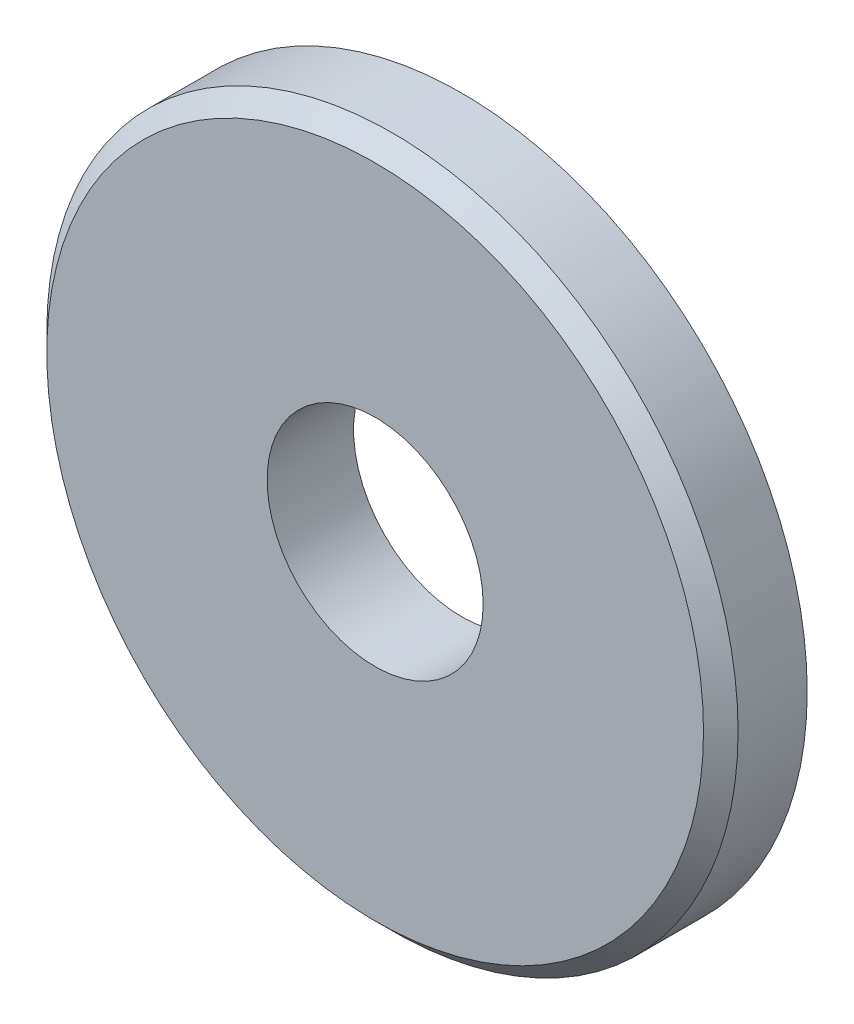
SolidWorks part; units mm, degrees
material "1023 碳钢板 (SS)"
ref_plane "前视基准面" through (0, 0, 0) normal (0, 0, 1) x (1, 0, 0)
ref_plane "上视基准面" through (0, 0, 0) normal (0, 1, 0) x (1, 0, 0)
ref_plane "右视基准面" through (0, 0, 0) normal (1, 0, 0) x (0, 0, -1)
sketch "草图1" plane through (0, 0, 0) normal (0, 0, 1) x (1, 0, 0)
  circle A0 centre (0, 0) radius 20
  circle A1 centre (0, 0) radius 6.25
  dimension "D1" = 40
  dimension "D2" = 12.5
extrude "凸台-拉伸1" add sketch "草图1" along normal blind 5
chamfer "倒角1" distance 1 angle 45 1 edges at (20, 0, 5)
